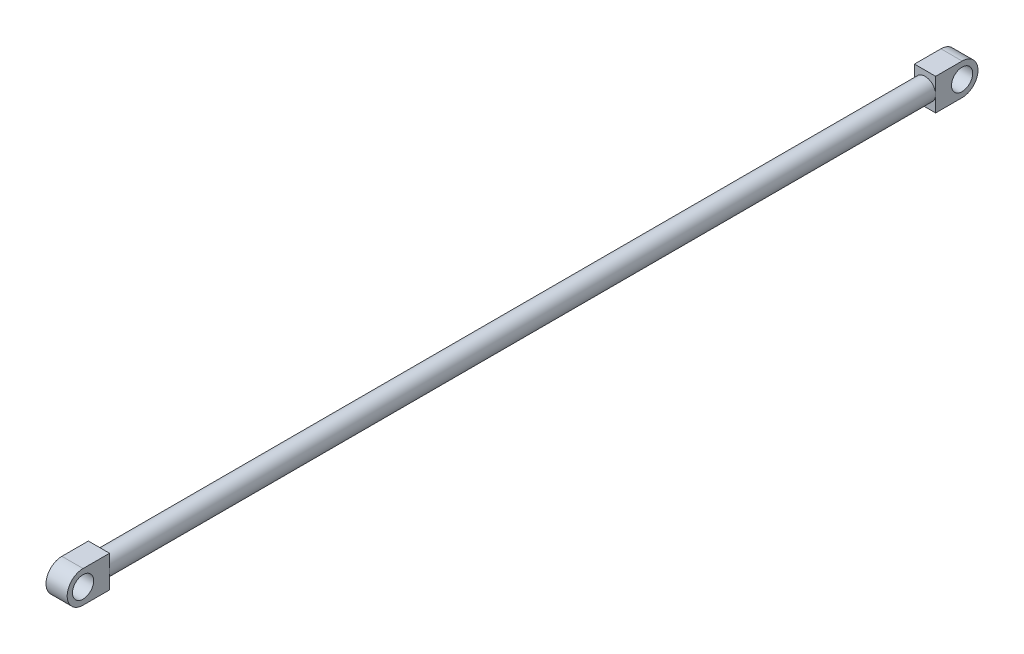
from build123d import *

# Parameters (mm, degrees)
SKETCH1_R           = 5
BOSS_EXTRUDE1_DEPTH = 390
SKETCH2_W           = 10
SKETCH2_H           = 15
BOSS_EXTRUDE2_DEPTH = 20
SKETCH3_W           = 10
SKETCH3_H           = 15
BOSS_EXTRUDE3_DEPTH = 20
SKETCH4_R           = 5
CUT_EXTRUDE1_DEPTH  = 411.190504522


with BuildPart() as part:
    # Sketch1 → Boss-Extrude1 (new body)
    with BuildSketch(Plane.XY):
        Circle(SKETCH1_R)
    extrude(amount=BOSS_EXTRUDE1_DEPTH)

    # Sketch2 → Boss-Extrude2 (add)
    with BuildSketch(Plane(origin=(0, 0, 0), x_dir=(-1, 0, 0), z_dir=(0, 0, -1))):
        Rectangle(SKETCH2_W, SKETCH2_H)
    extrude(amount=BOSS_EXTRUDE2_DEPTH)

    # Sketch3 → Boss-Extrude3 (add)
    with BuildSketch(Plane.XY.offset(390)):
        Rectangle(SKETCH3_W, SKETCH3_H)
    extrude(amount=BOSS_EXTRUDE3_DEPTH)

    # Sketch4 → Cut-Extrude1 (cut, through all)
    with BuildSketch(Plane(origin=(5, 0, 0), x_dir=(0, 0, -1), z_dir=(1, 0, 0))):
        with Locations((12.5, 0)):
            Circle(SKETCH4_R)
        with Locations((-402.5, 0)):
            Circle(SKETCH4_R)
        with BuildLine():
            Line((12.5, -7.5), (27.957175819, -19.344646022))
            Line((27.957175819, -19.344646022), (25.412525065, 11.111642689))
            Line((25.412525065, 11.111642689), (12.5, 7.5))
            ThreePointArc((12.5, 7.5), (20, 0), (12.5, -7.5))
        make_face()
        with BuildLine():
            Line((-402.5, 7.5), (-436.593003508, 16.998965127))
            Line((-436.593003508, 16.998965127), (-417.537871644, -29.426265233))
            Line((-417.537871644, -29.426265233), (-402.5, -7.5))
            ThreePointArc((-402.5, -7.5), (-410, 0), (-402.5, 7.5))
        make_face()
    extrude(amount=-CUT_EXTRUDE1_DEPTH, mode=Mode.SUBTRACT)


solid = part.part
